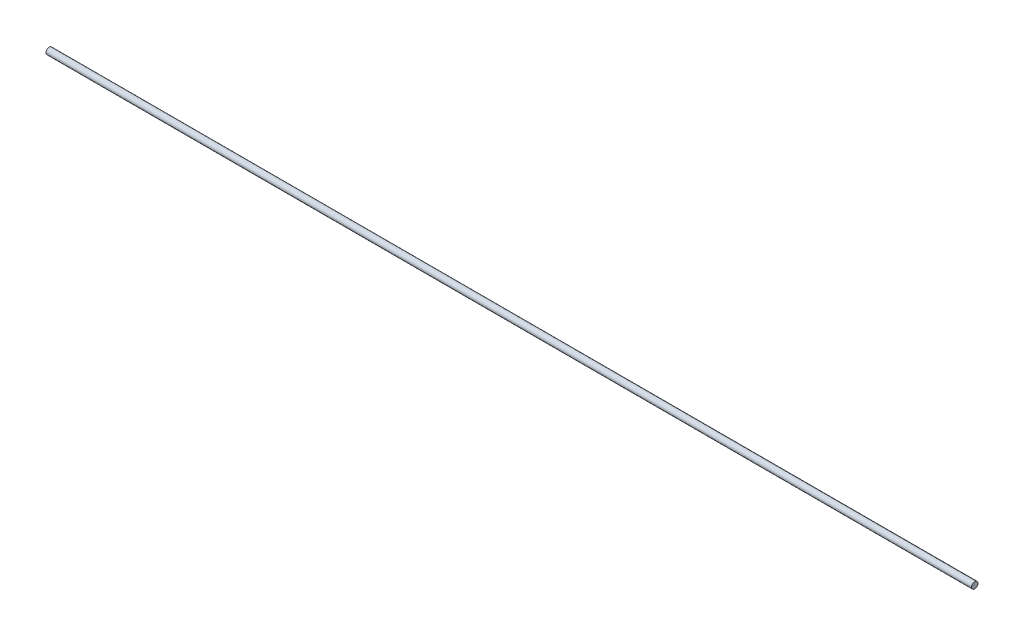
SolidWorks part; units mm, degrees
ref_plane "前视基准面" through (0, 0, 0) normal (0, 0, 1) x (1, 0, 0)
ref_plane "上视基准面" through (0, 0, 0) normal (0, 1, 0) x (1, 0, 0)
ref_plane "右视基准面" through (0, 0, 0) normal (1, 0, 0) x (0, 0, -1)
sketch "草图1" plane through (0, 0, 0) normal (0, 0, 1) x (1, 0, 0)
  line L0 (0, 50) -> (0, 45)
  line L1 (0, 45) -> (1440, 45)
  line L2 (1440, 45) -> (1440, 50)
  line L7 (1440, 50) -> (0, 50)
  line L8 (0, 45) -> (1440, 45) construction
  dimension "D3" = 1440
  dimension "D5" = 5
revolve "旋转1" add sketch "草图1" angle 360 about L8
cosmetic thread "装饰螺纹线1" parameters "D1"=350, "D2"=8.376
cosmetic thread "装饰螺纹线2" parameters "D1"=350, "D2"=6.647
